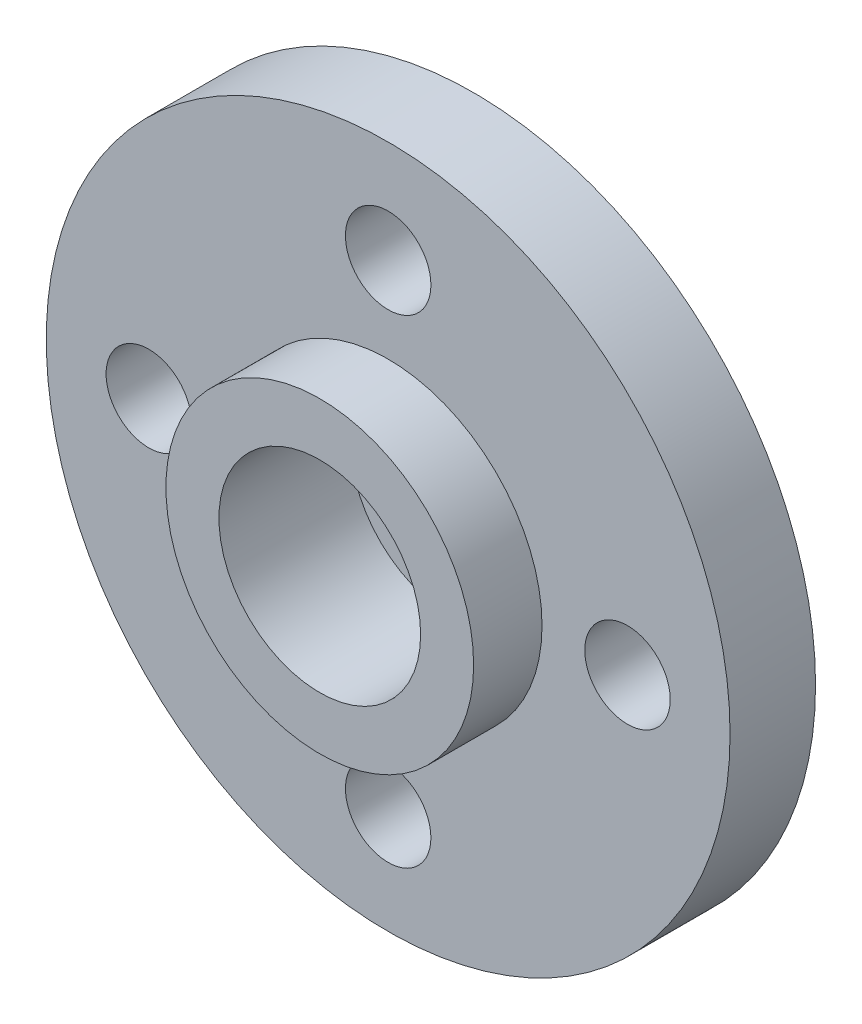
SolidWorks part; units mm, degrees
ref_plane "Front Plane" through (0, 0, 0) normal (0, 0, 1) x (1, 0, 0)
ref_plane "Top Plane" through (0, 0, 0) normal (0, 1, 0) x (1, 0, 0)
ref_plane "Right Plane" through (0, 0, 0) normal (1, 0, 0) x (0, 0, -1)
other "Configuration Table"
sketch "Sketch1" plane through (0, 0, 0) normal (0, 0, 1) x (1, 0, 0)
  circle A0 centre (0, 0) radius 10
  dimension "D1" = 20
extrude "Boss-Extrude1" add sketch "Sketch1" along normal blind 4.5
sketch "Sketch2" plane through (0, 0, 4.5) normal (0, 0, 1) x (1, 0, 0)
  circle A0 centre (0, 0) radius 10 construction
  circle A1 centre (0, 0) radius 10
  circle A2 centre (0, 0) radius 4.5
  dimension "D1" = 9
extrude "Cut-Extrude1" cut sketch "Sketch2" against normal blind 2
sketch "Sketch3" plane through (0, 0, 2.5) normal (0, 0, 1) x (1, 0, 0)
  line L0 (0, 0) -> (0, 10.4856) construction
  line L1 (0, 0) -> (-18.0519, 0) construction
  circle A0 centre (0, 7) radius 0.75
  circle A1 centre (7, 0) radius 0.75
  circle A2 centre (0, -7) radius 0.75
  circle A3 centre (-7, 0) radius 0.75
  point P15 (0, 0)
  dimension "D1" = 1.5
  dimension "D2" = 7
  dimension "D3" = 4
extrude "Cut-Extrude2" cut sketch "Sketch3" against normal through all
sketch "Sketch4" plane through (0, 0, 4.5) normal (0, 0, 1) x (1, 0, 0)
  circle A0 centre (0, 0) radius 2.95
  dimension "D1" = 5.9
extrude "Cut-Extrude3" cut sketch "Sketch4" against normal blind 3.85
sketch "Sketch5" plane through (0, 0, 0.65) normal (0, 0, 1) x (1, 0, 0)
  circle A0 centre (0, 0) radius 1.5
  dimension "D1" = 3
extrude "Cut-Extrude4" cut sketch "Sketch5" against normal through all
hole_wizard "M3 Tapped Hole2" positions "Sketch10" profile "Sketch11" tap size "M3" standard "GB" end condition through all
sketch "Sketch10" plane through (0, 0, 2.5) normal (0, 0, 1) x (1, 0, 0)
  point P0 (-7, 0)
  point P3 (0, 7)
  point P6 (7, 0)
  point P9 (0, -7)
sketch "Sketch11" plane through (-7, 0, 2.5) normal (1, 0, 0) x (0, -1, 0)
  line L0 (0, 0) -> (0, 2.5)
  line L1 (0, 2.5) -> (1.25, 2.5)
  line L2 (1.25, 2.5) -> (1.25, 0)
  line L5 (1.25, 0) -> (0, 0)
  line L11 (0, -6.35) -> (0, 107.95) construction
  dimension "通孔螺纹孔钻头直径" = 2.5
  dimension "通孔螺纹孔钻头深度" = 2.5
cosmetic thread "CosmeticThread5" parameters "D2"=3
cosmetic thread "CosmeticThread6" parameters "D2"=3
cosmetic thread "CosmeticThread7" parameters "D2"=3
cosmetic thread "CosmeticThread8" parameters "D2"=3
